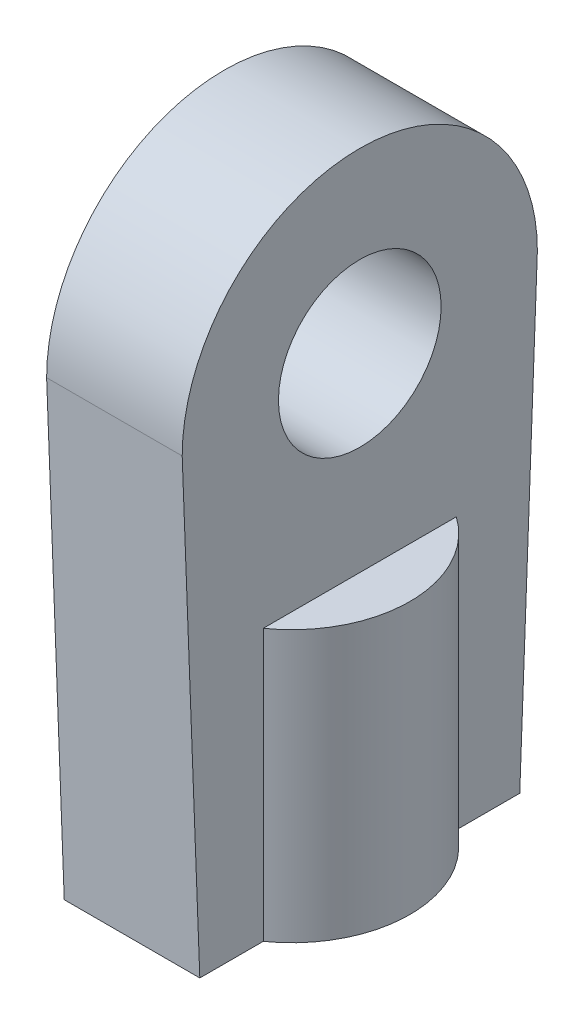
SolidWorks part; units mm, degrees
material "Q235B"
ref_plane "Front Plane" through (0, 0, 0) normal (0, 0, 1) x (1, 0, 0)
ref_plane "Top Plane" through (0, 0, 0) normal (0, 1, 0) x (1, 0, 0)
ref_plane "Right Plane" through (0, 0, 0) normal (1, 0, 0) x (0, 0, -1)
sketch "Sketch1" plane through (0, 0, 0) normal (1, 0, 0) x (0, 0, -1)
  line L0 (0, 170) -> (0, 0) construction
  line L1 (59, 0) -> (-59, 0)
  line L2 (-59, 0) -> (-65.5, 170)
  line L3 (59, 0) -> (65.5, 170)
  circle A0 centre (0, 170) radius 65.5
  circle A1 centre (0, 170) radius 30
  dimension "D1" = 131
  dimension "D4" = 60
  dimension "D2" = 170
  dimension "D3" = 118
extrude "Boss-Extrude1" add sketch "Sketch1" along normal mid plane 50
sketch "Sketch2" plane through (0, 0, 0) normal (0, 1, 0) x (1, 0, 0)
  circle A0 centre (0, 0) radius 43.5
  dimension "D1" = 87
extrude "Boss-Extrude2" add sketch "Sketch2" along normal blind 100
